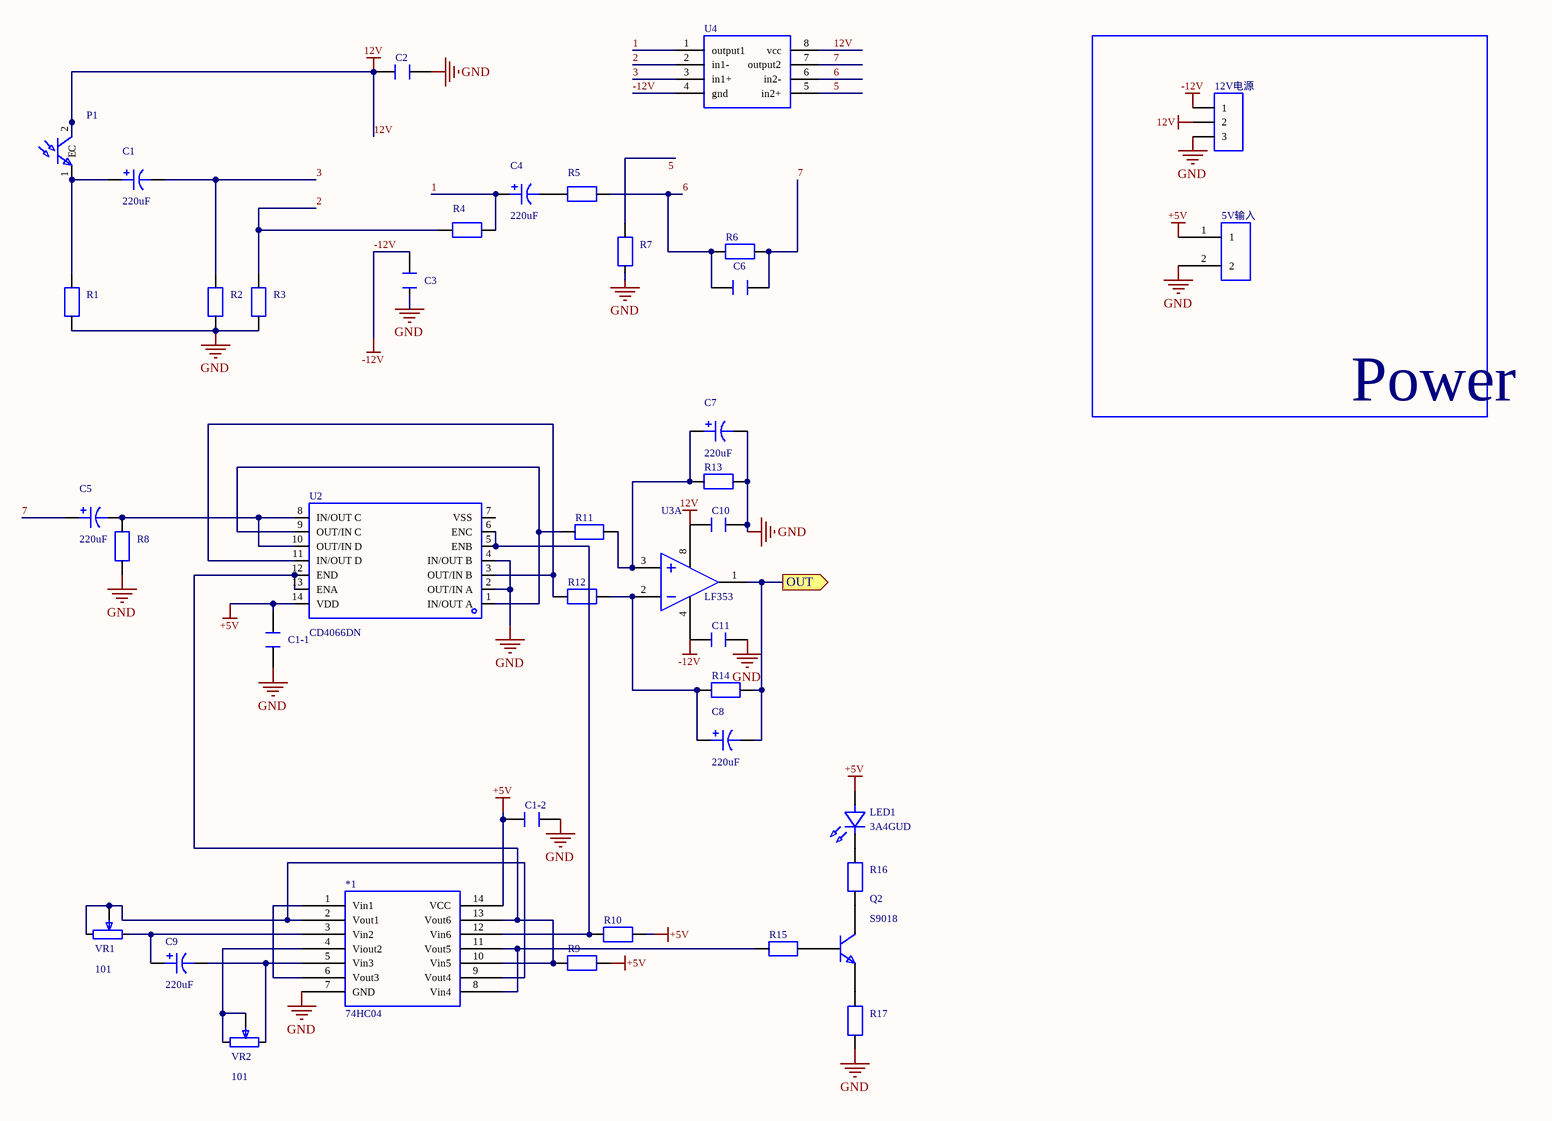
[diagram p0: MISC75396-3.schdoc]
# Altium project MISC75396-2.PrjPcb
1 sheet, 41 parts. Net scope: flat (ports and power ports of the same name join across sheets).
Board file: MISC75396.pcbdoc

## Sheet MISC75396-3.schdoc
size 420 x 297 mm; Version: V1.0; @Project Name: MISC75396; @Page Count: 1; @Update Date: 2026-03-14; @Create Date: 2026-03-14; @Schematic Name: MISC75396; @Page No: 1; @Board Name: MISC75396; @Create Time: 18:26:39; @Update Time: 23:54:28; Size: A4

### Parts
5V输入  5V output  [2INT]  (value not drawn)
12V电源  3PIN  [3PIN]  (value not drawn)
*1  74HC04  [DIP14]
C1  220uF  [CAP-TH_BD6.3-P2.50-D0.5-FD]
C1-1  (no value)  [电容直插]
C1-2  (no value)  [电容直插]
C2  (no value)  [电容直插]
C3  (no value)  [电容直插]
C4  220uF  [CAP-TH_BD6.3-P2.50-D0.5-FD]
C5  220uF  [CAP-TH_BD6.3-P2.50-D0.5-FD]
C6  (no value)  [电容直插]
C7  220uF  [CAP-TH_BD6.3-P2.50-D0.5-FD]
C8  220uF  [CAP-TH_BD6.3-P2.50-D0.5-FD]
C9  220uF  [CAP-TH_BD6.3-P2.50-D0.5-FD]
C10  (no value)  [电容直插]
C11  (no value)  [电容直插]
LED1  3A4GUD  [LED-TH_BD3.5-P2.54-RD-GREEN]
P1  (no value)  [LED_D3.0mm_Horizontal_O1.27mm_Z2.0mm]
Q2  S9018  [TO-92-3_L4.9-W3.7-P1.27-L]
R1  (no value)  [D45-V(直插)]
R2  (no value)  [D45-V(直插)]
R3  (no value)  [D45-V(直插)]
R4  (no value)  [D45-V(直插)]
R5  (no value)  [D45-V(直插)]
R6  (no value)  [D45-V(直插)]
R7  (no value)  [D45-V(直插)]
R8  (no value)  [D45-V(直插)]
R9  (no value)  [D45-V(直插)]
R10  (no value)  [D45-V(直插)]
R11  (no value)  [D45-V(直插)]
R12  (no value)  [D45-V(直插)]
R13  (no value)  [D45-V(直插)]
R14  (no value)  [D45-V(直插)]
R15  (no value)  [D45-V(直插)]
R16  (no value)  [D45-V(直插)]
R17  (no value)  [D45-V(直插)]
U2  CD4066DN  [PDIP-14_L19.3-W6.5-P2.54-LS7.6-BL]
U3  LF353  [DIP-8]  (part A of 2)
U4  (no value)  [DIP-8_L9.9-W6.4-P2.54-LS7.6-BL]
VR1  101  [3296W]
VR2  101  [3296W]

### Blocks framed on the sheet
Power: 5V输入 12V电源

### Ports
OUT (out)

### Nets
12V: 12V电源.2 C2.2 C10.2 P1.2(C) U3.8(V+) U4.8(vcc)
+5V: 5V输入.1 *1.14(VCC) C1-1.2 C1-2.2 LED1.2(A) R9.2 R10.2 U2.14(VDD)
-12V: 12V电源.1 C3.2 C11.2 U3.4(V-) U4.4(gnd)
GND: 5V输入.2 12V电源.3 *1.7(GND) C1-1.1 C1-2.1 C2.1 C3.1 C7.2 C10.1 C11.1 R1.2 R2.2 R3.2 R7.1 R8.2 R13.2 R17.1 U2.2(OUT/IN_A) U2.4(IN/OUT_B)
1: C4.1 R4.1 U4.1(output1)
2: R3.1 R4.2 U4.2(in1-)
3: C1.2 R2.1 U4.3(in1+)
5: R7.2 U4.5(in2+)
6: C6.2 R5.1 R6.1 U4.6(in2-)
7: C5.1 C6.1 R6.2 U4.7(output2)
Net*1_1: *1.1(Vin1) *1.6(Vout3)
Net*1_2: *1.2(Vout1) *1.9(Vout4) VR1.1 VR1.2
Net*1_3: *1.3(Vin2) C9.1 VR1.3
Net*1_4: *1.4(Viout2) VR2.1 VR2.2
Net*1_5: *1.5(Vin3) C9.2 VR2.3
Net*1_8: *1.8(Vin4) *1.11(Vout5) R15.1
Net*1_10: *1.10(Vin5) *1.13(Vout6) R9.1 U2.12(END) U2.13(ENA)
Net*1_12: *1.12(Vin6) R10.1 U2.5(ENB) U2.6(ENC)
NetC1_1: C1.1 P1.1(E) R1.1
NetC4_2: C4.2 R5.2
NetC5_2: C5.2 R8.1 U2.8(IN/OUT_C) U2.10(OUT/IN_D)
NetC7_1: C7.1 R11.2 R13.1 U3.3(IN+)
NetC8_1: C8.1 R12.2 R14.1 U3.2(IN-)
NetC8_2: C8.2 R14.2 U3.1(OUT) ; port OUT
NetLED1_1: LED1.1(C) R16.2
NetQ2_1: Q2.1(E) R17.2
NetQ2_2: Q2.2(B) R15.2
NetQ2_3: Q2.3(C) R16.1
NetR11_1: R11.1 U2.1(IN/OUT_A) U2.9(OUT/IN_C)
NetR12_1: R12.1 U2.3(OUT/IN_B) U2.11(IN/OUT_D)

Not connected (* = marked no-connect by the designer): U2 7(VSS)

### Notes on the sheet
- 2026-03-14
- Schematic
- Board
- Sheet
- P1
- Drawn
- Reviewed
- Project file
- Revision
- Size
- A4
- page 1 Total 1

### Library data of the parts
5V输入 = 2PIN: AddInBom: yes; Device: 2PIN; ConvertToPcb: yes; SymbolName: 2PIN; Origin Footprint 2: 2INT; FootprintName: 2INT
12V电源 = 3PIN: Origin Footprint 2: 1*3PIN; AddInBom: yes; Device: 3PIN; Origin Footprint 3: 3PIN; Origin Footprint 4: 1*3PIN; Origin Footprint 5: 1*3PIN; ConvertToPcb: yes; SymbolName: 1*3PIN; FootprintName: 3PIN
*1 = 74HC04: AddInBom: yes; _: 3; Device: 74HC04; ConvertToPcb: yes; SymbolName: 74HC04; FootprintName: DIP14
C1 C4 C5 C7-C9 = ERG16V220M6X7: Capacitance: 220uF; tolerance: ±20%; rated voltage: 16V; ripple current: 300mA@100kHz; equivalent series resistance (ESR): 220mΩ@100kHz;; Manufacturer: JIERR(捷而瑞); AddInBom: yes; ModelId: 983aa343eddc42b59ebb10541a88166e; ModelTransform: 247.99486,248.229,0,90,0,0,0,0,-196.85; Pin Spacing: 2.5mm; Lifetime: 2000hrs@105℃; Symbol: ERG16V220M6X7; Device: ERG16V220M6X7; LCSC Part Name: 220uF ±20% 16V; SupplierPart: C47344172; ManufacturerPart: ERG16V220M6X7; Supplier Footprint: 插件,D6.3xL7mm; JLCPCB Part Class: Extended library; Datasheet: https://item.szlcsc.com/datasheet/ERG16V220M6X7/49556613.html; Supplier: LCSC; ConvertToPcb: yes; FootprintName: CAP-TH_BD6.3-P2.50-D0.5-FD; ModelName: CAP-TH_BD6.3-P2.50-D0.5-FD; Value: 220uF; Tolerance: ±20%; Voltage Rating: 16V; Ripple Current: 300mA@100kHz; Equivalent Series Resistance(ESR): 220mΩ@100kHz; Diameter: 6mm; Height - Seated (Max): 7mm; Operating Temperature: -40℃~+105℃
C1-1 C1-2 C2 C3 C6 C10 C11 = 电容直插: Device: Through-hole capacitor; AddInBom: yes; ModelId: 85437cda0c2b439094ae87a6c0e47ecb; ModelName: Ceramic capacitor; ModelTransform: 222.82,98.42,339.54,0,0,0,0,0,-39.37; ConvertToPcb: yes; SymbolName: Through-hole capacitor; FootprintName: Through-hole capacitor
LED1 = 3A4GUD: Lamp holder type: 3mm round lamp holder; luminous colour: emerald green; forward voltage drop (Vf): 2.8V~3.2V; forward current: 20mA; wavelength: 520nm~525nm; lens colour: green lens; colour temperature: -; luminous intensity: 8000mcd~12000mcd; viewing angle: 30°; operating temperature: -40℃~+85℃;; Manufacturer: Guiguang light(桂光光电); AddInBom: yes; ModelId: 00abdbf2c53742c78999362c055e6c63; ModelTransform: 130.31911,137.754,0,180,0,0,3.15,0,-196.85; Peak Wavelength: 525nm; Symbol: 3A4GUD; Device: 3A4GUD; LCSC Part Name: 3mm 绿发翠绿长脚; SupplierPart: C52034646; ManufacturerPart: 3A4GUD; Supplier Footprint: 插件,D=3mm; JLCPCB Part Class: Extended library; Datasheet: https://item.szlcsc.com/datasheet/3A4GUD/54791014.html; Supplier: LCSC; ConvertToPcb: yes; FootprintName: LED-TH_BD3.5-P2.54-RD-GREEN; ModelName: LED-TH_BD3.5-P2.54-RD-GREEN; Lamp Holder Type: 3mm round lamp holder; Illumination Color: Emerald green; Voltage - Forward(Vf): 2.8V~3.2V; Forward Current: 20mA; Wavelength - Dominant: 520nm~525nm; Lens Color: Green lens; Color Temperature: -; Luminous Intensity: 8000mcd~12000mcd; Viewing Angle: 30°; Operating Temperature: -40℃~+85℃
P1 = LED-3MM-红外接收: Symbol: LED2; Device: LED-3MM-infrared receiver; ConvertToPcb: yes; ModelId: 02bfc7c664ed44c69e400cbfd76bc52c; ModelTransform: 135,267.28,229.29,0,0,0,57.5,-122,-100; Value: 红外接收; AddInBom: yes; FootprintName: LED_D3.0mm_Horizontal_O1.27mm_Z2.0mm; ModelName: LED_D3.0mm_Horizontal_O1.27mm_Z2.0mm
Q2 = S9018: Transistor type: NPN; collector-emitter breakdown voltage (Vceo): 18V; collector current (Ic): 50mA; power (Pd): 400mW; collector cut-off current (Icbo): 100nA; collector-emitter saturation voltage (VCE(sat)@Ic,Ib): 500mV@10mA,1mA; DC current gain (hFE@Ic,Vce): 97@1mA,5V; transition frequency (fT): 800MHz; operating temperature: +150℃@(Tj);; Manufacturer: CJ(江苏长电/长晶); AddInBom: yes; ModelId: aafe8e06f2154e7c93506efd0d6632dd; ModelTransform: 180.7872,141.4455,0,0,0,0,0,22.677,-196.85; Device: S9018; ConvertToPcb: yes; SymbolName: S9018; LCSC Part Name: NPN 18V 50mA H档97-146; SupplierPart: C78893; ManufacturerPart: S9018; Supplier Footprint: TO-92-3; JLCPCB Part Class: Extended Part; Datasheet: https://atta.szlcsc.com/upload/public/pdf/source/20160723/1469258983703.pdf; Supplier: LCSC; ModelName: TO-92-3_L4.9-W3.7-P1.27-L; Transistor Type: NPN; Collector-Emitter Breakdown Voltage (Vceo): 18V; Collector Current (Ic): 50mA; Power Dissipation (Pd): 400mW; Collector Cut-Off Current (Icbo): 100nA; Collector-Emitter Saturation Voltage (VCE(sat)@Ic,Ib): 500mV@10mA,1mA; DC Current Gain (hFE@Ic,Vce): 97@1mA,5V; Transition Frequency (fT): 800MHz; Operating Temperature: +150℃@(Tj); FootprintName: TO-92-3_L4.9-W3.7-P1.27-L
R1-R17 = 直插电阻: Through-hole resistor; AddInBom: yes; ModelId: 01fe6002a9f04defb2675523a429ba7d; ModelName: Axial_4_0x11_0_Vert; ModelTransform: 992.24408708925,358.65377,210.36173682434887,0,90,90,43.30709,102.3622,299.2126; Device: Through-hole resistor; ConvertToPcb: yes; SymbolName: Through-hole resistor; FootprintName: D45-V (through-hole)
U2 = CD4066DN: Switch circuit: 1:1; channels: 4; on-resistance (Ron): 125Ω;; Manufacturer: HGSEMI(华冠); AddInBom: yes; ModelId: 7604059b31ae49f98a0332a7cce2343e; ModelTransform: 759.15391,311.417,0,0,0,0,0,0,-129.921; Number of Channels: 4; Voltage - Supply: 3V~15V; Propagation Delay (tpd): 15ns; Symbol: CD4066DN; Device: CD4066DN; LCSC Part Name: CD4066DN; SupplierPart: C42406219; ManufacturerPart: CD4066DN; Supplier Footprint: DIP-14; Datasheet: https://item.szlcsc.com/datasheet/CD4066DN/44377199.html; Supplier: LCSC; ConvertToPcb: yes; FootprintName: PDIP-14_L19.3-W6.5-P2.54-LS7.6-BL; ModelName: PDIP-14_L19.3-W6.5-P2.54-LS7.6-BL; Switch Circuit: 1:1; Turn-on time: -; Ron: 125Ω; Turn-off time: -; Operating Temperature: -20℃~+85℃
U3 = LF353: Relevance: []; AddInBom: yes; ModelId: b25ce56d62334bb48ac4eeaf82c54c81; Device: LF353; LatestRevisionDate: 2023; ConvertToPcb: yes; SymbolName: LF353; FootprintName: DIP-8; ModelName: DIP-8; Publisher: hjh
U4 = lf353: AddInBom: yes; Device: lf353; ConvertToPcb: yes; SymbolName: lf353
VR1 VR2 = 3296: AddInBom: yes; Origin Footprint 2: 103; ModelId: b182808559bb43bda9e7de64b64134cb; Device: 3296; ConvertToPcb: yes; SymbolName: 3296; FootprintName: 3296W; ModelName: 3296W